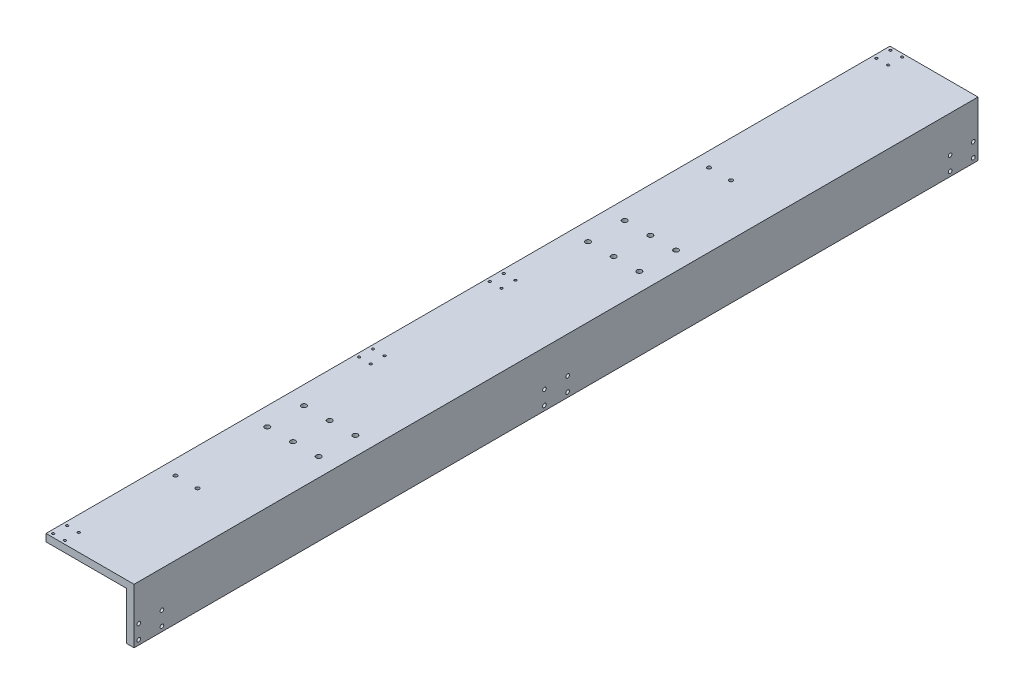
SolidWorks part; units mm, degrees
material "6061Al"
ref_plane "前视基准面" through (0, 0, 0) normal (0, 0, 1) x (1, 0, 0)
ref_plane "上视基准面" through (0, 0, 0) normal (0, 1, 0) x (1, 0, 0)
ref_plane "右视基准面" through (0, 0, 0) normal (1, 0, 0) x (0, 0, -1)
sketch "草图1" plane through (0, 0, 0) normal (0, 0, 1) x (1, 0, 0)
  line L0 (0, 0) -> (120, 0)
  line L1 (120, 0) -> (120, -75)
  line L2 (0, -10) -> (110, -10)
  line L3 (110, -10) -> (110, -75)
  line L4 (0, 0) -> (0, -10)
  line L5 (110, -75) -> (120, -75)
  dimension "D1" = 120
  dimension "D2" = 75
  dimension "D3" = 10
extrude "凸台-拉伸1" add sketch "草图1" along normal mid plane 1150
hole_wizard "M4 螺纹孔1" positions "草图2" profile "草图3" tap size "M4" standard "ISO" end condition through all
sketch "草图2" plane through (0, 0, 0) normal (0, 1, 0) x (1, 0, 0)
  point P0 (5.2, 43.6)
  point P3 (21.1, 43.6)
  point P6 (5.2, 24.6)
  point P9 (21.1, 24.6)
  point P12 (5.2, -134.6)
  point P15 (21.1, -134.6)
  point P18 (5.2, -153.6)
  point P21 (21.1, -153.6)
  point P24 (5.2, -551.4)
  point P27 (21.1, -551.4)
  point P30 (5.2, -570.4)
  point P33 (21.1, -570.4)
  point P36 (5.2, 570.4)
  point P39 (21.1, 570.4)
  point P42 (21.1, 551.4)
  point P45 (5.2, 551.4)
sketch "草图3" plane through (5.2, 0, -43.6) normal (1, 0, 0) x (0, 0, 1)
  line L0 (0, 0) -> (0, 75)
  line L1 (0, 75) -> (1.65, 75)
  line L2 (1.65, 75) -> (1.65, 0)
  line L5 (1.65, 0) -> (0, 0)
  line L11 (0, -6.35) -> (0, 107.95) construction
  dimension "通孔螺纹孔钻头直径" = 3.3
  dimension "通孔螺纹孔钻头深度" = 75
cosmetic thread "孔螺蚊线1" parameters "D2"=4
cosmetic thread "孔螺蚊线2" parameters "D2"=4
cosmetic thread "孔螺蚊线3" parameters "D2"=4
cosmetic thread "孔螺蚊线4" parameters "D2"=4
cosmetic thread "孔螺蚊线5" parameters "D2"=4
cosmetic thread "孔螺蚊线6" parameters "D2"=4
cosmetic thread "孔螺蚊线7" parameters "D2"=4
cosmetic thread "孔螺蚊线8" parameters "D2"=4
cosmetic thread "孔螺蚊线9" parameters "D2"=4
cosmetic thread "孔螺蚊线10" parameters "D2"=4
cosmetic thread "孔螺蚊线11" parameters "D2"=4
cosmetic thread "孔螺蚊线12" parameters "D2"=4
cosmetic thread "孔螺蚊线13" parameters "D2"=4
cosmetic thread "孔螺蚊线14" parameters "D2"=4
cosmetic thread "孔螺蚊线15" parameters "D2"=4
cosmetic thread "孔螺蚊线16" parameters "D2"=4
hole_wizard "M6 螺纹孔1" positions "草图4" profile "草图5" tap size "M6" standard "ISO" end condition through all
sketch "草图4" plane through (0, 0, 0) normal (0, 1, 0) x (1, 0, 0)
  line L0 (0, -575) -> (0, 575) construction
  line L1 (120, -575) -> (0, -575) construction
  line L2 (120, 575) -> (0, 575) construction
  point P0 (20, 308.5)
  point P3 (50, 308.5)
  point P6 (20, -418.5)
  point P9 (50, -418.5)
  dimension "D1" = 30
  dimension "D2" = 20
  dimension "D3" = 156.5
  dimension "D4" = 266.5
sketch "草图5" plane through (20, 0, -308.5) normal (1, 0, 0) x (0, 0, 1)
  line L0 (0, 0) -> (0, 75)
  line L1 (0, 75) -> (2.5, 75)
  line L2 (2.5, 75) -> (2.5, 0)
  line L5 (2.5, 0) -> (0, 0)
  line L11 (0, -6.35) -> (0, 107.95) construction
  dimension "通孔螺纹孔钻头直径" = 5
  dimension "通孔螺纹孔钻头深度" = 75
cosmetic thread "孔螺蚊线17" parameters "D2"=6
cosmetic thread "孔螺蚊线18" parameters "D2"=6
cosmetic thread "孔螺蚊线48" parameters "D2"=6
cosmetic thread "孔螺蚊线49" parameters "D2"=6
hole_wizard "M8 螺纹孔1" positions "草图6" profile "草图7" tap size "M8" standard "ISO" end condition through all
sketch "草图6" plane through (0, 0, 0) normal (0, 1, 0) x (1, 0, 0)
  point P0 (25, 188.5)
  point P3 (60, 188.5)
  point P6 (95, 188.5)
  point P9 (95, 138.5)
  point P12 (60, 138.5)
  point P15 (25, 138.5)
  point P18 (25, -248.5)
  point P21 (60, -248.5)
  point P24 (95, -248.5)
  point P27 (95, -298.5)
  point P30 (60, -298.5)
  point P33 (25, -298.5)
sketch "草图7" plane through (25, 0, -188.5) normal (1, 0, 0) x (0, 0, 1)
  line L0 (0, 0) -> (0, 75)
  line L1 (0, 75) -> (3.4, 75)
  line L2 (3.4, 75) -> (3.4, 0)
  line L5 (3.4, 0) -> (0, 0)
  line L11 (0, -6.35) -> (0, 107.95) construction
  dimension "通孔螺纹孔钻头直径" = 6.8
  dimension "通孔螺纹孔钻头深度" = 75
cosmetic thread "孔螺蚊线22" parameters "D2"=8
cosmetic thread "孔螺蚊线23" parameters "D2"=8
cosmetic thread "孔螺蚊线24" parameters "D2"=8
cosmetic thread "孔螺蚊线25" parameters "D2"=8
cosmetic thread "孔螺蚊线28" parameters "D2"=8
cosmetic thread "孔螺蚊线29" parameters "D2"=8
cosmetic thread "孔螺蚊线30" parameters "D2"=8
cosmetic thread "孔螺蚊线31" parameters "D2"=8
cosmetic thread "孔螺蚊线50" parameters "D2"=8
cosmetic thread "孔螺蚊线51" parameters "D2"=8
cosmetic thread "孔螺蚊线52" parameters "D2"=8
cosmetic thread "孔螺蚊线53" parameters "D2"=8
hole_wizard "M6 螺纹孔2" positions "草图8" profile "草图9" tap size "M6" standard "ISO" end condition through all
sketch "草图8" plane through (120, 0, 0) normal (1, 0, 0) x (0, 0, -1)
  point P0 (-568.6, -49.6)
  point P3 (-537, -49.6)
  point P6 (-537, -49.6)
  point P8 (-537, -68.6)
  point P11 (-568.6, -68.6)
  point P14 (-15.8, -49.6)
  point P17 (15.8, -49.6)
  point P20 (15.8, -68.6)
  point P23 (-15.8, -68.6)
  point P26 (537, -49.6)
  point P29 (568.6, -49.6)
  point P32 (568.6, -68.6)
  point P35 (537, -68.6)
sketch "草图9" plane through (120, -49.6, 568.6) normal (0, 1, 0) x (0, 0, -1)
  line L0 (0, 0) -> (0, 120)
  line L1 (0, 120) -> (2.5, 120)
  line L2 (2.5, 120) -> (2.5, 0)
  line L5 (2.5, 0) -> (0, 0)
  line L11 (0, -6.35) -> (0, 107.95) construction
  dimension "通孔螺纹孔钻头直径" = 5
  dimension "通孔螺纹孔钻头深度" = 120
cosmetic thread "孔螺蚊线33" parameters "D2"=6
cosmetic thread "孔螺蚊线34" parameters "D2"=6
cosmetic thread "孔螺蚊线35" parameters "D2"=6
cosmetic thread "孔螺蚊线36" parameters "D2"=6
cosmetic thread "孔螺蚊线37" parameters "D2"=6
cosmetic thread "孔螺蚊线38" parameters "D2"=6
cosmetic thread "孔螺蚊线39" parameters "D2"=6
cosmetic thread "孔螺蚊线40" parameters "D2"=6
cosmetic thread "孔螺蚊线41" parameters "D2"=6
cosmetic thread "孔螺蚊线42" parameters "D2"=6
cosmetic thread "孔螺蚊线44" parameters "D2"=6
cosmetic thread "孔螺蚊线45" parameters "D2"=6
